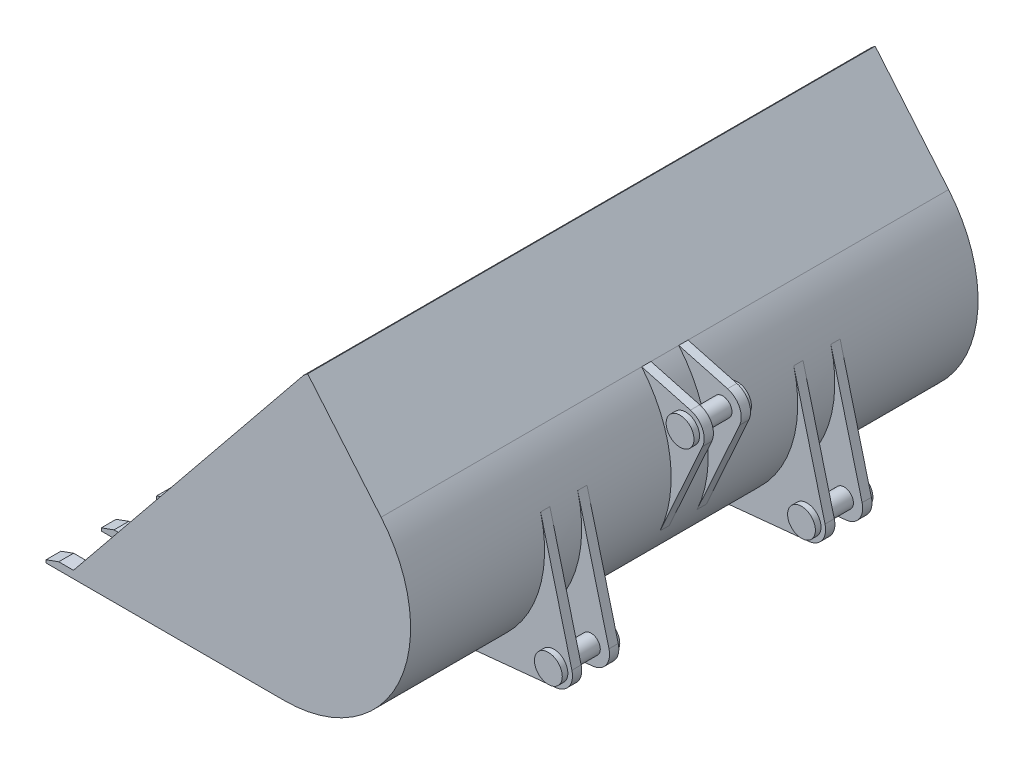
from build123d import *

# Parameters (mm, degrees)
BOSS_EXTRUDE1_DEPTH  = 3000
BOSS_EXTRUDE2_START  = 30
BOSS_EXTRUDE2_DEPTH  = 30
BOSS_EXTRUDE4_START  = -3000
BOSS_EXTRUDE4_DEPTH  = 30
BOSS_EXTRUDE5_START  = -692.5
SKETCH_1_11_R        = 50
BOSS_EXTRUDE5_DEPTH  = 50
BOSS_EXTRUDE6_START  = -892.5
SKETCH_1_12_R        = 50
BOSS_EXTRUDE6_DEPTH  = 50
BOSS_EXTRUDE7_START  = -1375
SKETCH_1_13_2_R      = 50
BOSS_EXTRUDE7_DEPTH  = 50
SKETCH_3_5_R         = 50
BOSS_EXTRUDE8_DEPTH  = 250
BOSS_EXTRUDE9_START  = 30
SKETCH_3_4_R         = 75
SKETCH_3_4_R_2       = 50
BOSS_EXTRUDE9_DEPTH  = 30
BOSS_EXTRUDE10_START = -250
SKETCH_3_5_2_R       = 75
SKETCH_3_5_2_R_2     = 50
BOSS_EXTRUDE10_DEPTH = 30
BOSS_EXTRUDE11_START = 30
SKETCH_4_3_R         = 75
SKETCH_4_3_R_2       = 50
BOSS_EXTRUDE11_DEPTH = 30
SKETCH_4_3_2_R       = 50
BOSS_EXTRUDE12_DEPTH = 125
BOSS_EXTRUDE13_DEPTH = 80
LPATTERN1_COUNT      = 11
LPATTERN1_PITCH      = 298


with BuildPart() as part:
    # Sketch 1_13 → Boss-Extrude1 (new body)
    with BuildSketch(Plane.XY):
        with BuildLine():
            ThreePointArc((1666.98072299, 1087.095574587), (1762.359796854, 362.619582016), (1146.070501669, -30))
            Line((1146.070501669, -30), (0, -30))
            Line((0, -30), (0, 0))
            Line((0, 0), (1146.070501669, 0))
            ThreePointArc((1146.070501669, 0), (1735.170563243, 375.298129869), (1643.999389696, 1067.811946296))
            Line((1643.999389696, 1067.811946296), (1247.99690453, 1539.749330669))
            Line((1247.99690453, 1539.749330669), (1270.978237824, 1559.03295896))
            Line((1270.978237824, 1559.03295896), (1666.98072299, 1087.095574587))
        make_face()
    extrude(amount=-BOSS_EXTRUDE1_DEPTH)

    # 草图1<7> → Boss-Extrude2 (add)
    with BuildSketch(Plane.XY.offset(BOSS_EXTRUDE2_START)):
        with BuildLine():
            Line((1247.99690453, 1539.749330669), (0, 0))
            Line((0, 0), (0, -30))
            Line((0, -30), (1146.070501669, -30))
            ThreePointArc((1146.070501669, -30), (1762.359796854, 362.619582016), (1666.98072299, 1087.095574587))
            Line((1666.98072299, 1087.095574587), (1270.978237824, 1559.03295896))
            Line((1270.978237824, 1559.03295896), (1247.99690453, 1539.749330669))
        make_face()
    extrude(amount=-BOSS_EXTRUDE2_DEPTH)

    # 草图1<9> → Boss-Extrude4 (add)
    with BuildSketch(Plane.XY.offset(BOSS_EXTRUDE4_START)):
        with BuildLine():
            ThreePointArc((1643.999389696, 1067.811946296), (1735.170563243, 375.298129869), (1146.070501669, 0))
            Line((1146.070501669, 0), (0, 0))
            Line((0, 0), (1247.99690453, 1539.749330669))
            Line((1247.99690453, 1539.749330669), (1643.999389696, 1067.811946296))
        make_face()
        with BuildLine():
            ThreePointArc((1666.98072299, 1087.095574587), (1762.359796854, 362.619582016), (1146.070501669, -30))
            Line((1146.070501669, -30), (0, -30))
            Line((0, -30), (0, 0))
            Line((0, 0), (1146.070501669, 0))
            ThreePointArc((1146.070501669, 0), (1735.170563243, 375.298129869), (1643.999389696, 1067.811946296))
            Line((1643.999389696, 1067.811946296), (1247.99690453, 1539.749330669))
            Line((1247.99690453, 1539.749330669), (1270.978237824, 1559.03295896))
            Line((1270.978237824, 1559.03295896), (1666.98072299, 1087.095574587))
        make_face()
    extrude(amount=-BOSS_EXTRUDE4_DEPTH)

    # 草图1<11> → Boss-Extrude5 (add)
    with BuildSketch(Plane.XY.offset(BOSS_EXTRUDE5_START)):
        with BuildLine():
            Line((1213.095596051, -26.688729567), (1886.256631527, 39.986951534))
            ThreePointArc((1886.256631527, 39.986951534), (1958.361695899, 82.208810404), (1973.242532996, 164.430379118))
            Line((1973.242532996, 164.430379118), (1804.599726039, 819.526578004))
            ThreePointArc((1804.599726039, 819.526578004), (1703.410033783, 260.419910747), (1213.095596051, -26.688729567))
        make_face()
        with Locations((1876.4, 139.5)):
            Circle(SKETCH_1_11_R, mode=Mode.SUBTRACT)
    boss_extrude5 = extrude(amount=-BOSS_EXTRUDE5_DEPTH)

    # 草图1<12> → Boss-Extrude6 (add)
    with BuildSketch(Plane.XY.offset(BOSS_EXTRUDE6_START)):
        with BuildLine():
            Line((1213.095596051, -26.688729567), (1886.256631527, 39.986951534))
            ThreePointArc((1886.256631527, 39.986951534), (1958.361695899, 82.208810404), (1973.242532996, 164.430379118))
            Line((1973.242532996, 164.430379118), (1804.599726039, 819.526578004))
            ThreePointArc((1804.599726039, 819.526578004), (1703.410033783, 260.419910747), (1213.095596051, -26.688729567))
        make_face()
        with Locations((1876.4, 139.5)):
            Circle(SKETCH_1_12_R, mode=Mode.SUBTRACT)
    boss_extrude6 = extrude(amount=-BOSS_EXTRUDE6_DEPTH)

    # Sketch 1_13 2 → Boss-Extrude7 (add)
    with BuildSketch(Plane.XY.offset(BOSS_EXTRUDE7_START)):
        with BuildLine():
            Line((1930.061378111, 1016.371252693), (1666.98072299, 1087.095574587))
            ThreePointArc((1666.98072299, 1087.095574587), (1819.685246249, 742.968682279), (1765.902974507, 370.343593645))
            Line((1765.902974507, 370.343593645), (1995.251834241, 878.674057889))
            ThreePointArc((1995.251834241, 878.674057889), (1994.482550811, 962.590121629), (1930.061378111, 1016.371252693))
        make_face()
        with Locations((1904.1, 919.8)):
            Circle(SKETCH_1_13_2_R, mode=Mode.SUBTRACT)
    boss_extrude7 = extrude(amount=-BOSS_EXTRUDE7_DEPTH)

    # Sketch 3_5 → Boss-Extrude8 (add)
    with BuildSketch(Plane.XY.offset(-692.5)):
        with Locations((1876.4, 139.5)):
            Circle(SKETCH_3_5_R)
    boss_extrude8 = extrude(amount=-BOSS_EXTRUDE8_DEPTH)

    # 草图3<4> → Boss-Extrude9 (add)
    # profile 1 of 2: a face of its own
    with BuildSketch(Plane.XY.offset(-692.5).offset(BOSS_EXTRUDE9_START)):
        with Locations((1876.4, 139.5)):
            Circle(SKETCH_3_4_R)
        with Locations((1876.4, 139.5)):
            Circle(SKETCH_3_4_R_2, mode=Mode.SUBTRACT)
    # profile 2 of 2: a face of its own
    with BuildSketch(Plane.XY.offset(-692.5).offset(BOSS_EXTRUDE9_START)):
        with Locations((1876.4, 139.5)):
            Circle(SKETCH_3_4_R_2)
    boss_extrude9 = extrude(amount=-BOSS_EXTRUDE9_DEPTH)

    # Sketch 3_5 2 → Boss-Extrude10 (add)
    # profile 1 of 2: a face of its own
    with BuildSketch(Plane.XY.offset(-692.5).offset(BOSS_EXTRUDE10_START)):
        with Locations((1876.4, 139.5)):
            Circle(SKETCH_3_5_2_R)
        with Locations((1876.4, 139.5)):
            Circle(SKETCH_3_5_2_R_2, mode=Mode.SUBTRACT)
    # profile 2 of 2: a face of its own
    with BuildSketch(Plane.XY.offset(-692.5).offset(BOSS_EXTRUDE10_START)):
        with Locations((1876.4, 139.5)):
            Circle(SKETCH_3_5_2_R_2)
    boss_extrude10 = extrude(amount=-BOSS_EXTRUDE10_DEPTH)

    # Sketch 4_3 → Boss-Extrude11 (add)
    # profile 1 of 2: a face of its own
    with BuildSketch(Plane.XY.offset(-1375).offset(BOSS_EXTRUDE11_START)):
        with Locations((1904.1, 919.8)):
            Circle(SKETCH_4_3_R)
        with Locations((1904.1, 919.8)):
            Circle(SKETCH_4_3_R_2, mode=Mode.SUBTRACT)
    # profile 2 of 2: a face of its own
    with BuildSketch(Plane.XY.offset(-1375).offset(BOSS_EXTRUDE11_START)):
        with Locations((1904.1, 919.8)):
            Circle(SKETCH_4_3_R_2)
    boss_extrude11 = extrude(amount=-BOSS_EXTRUDE11_DEPTH)

    # Sketch 4_3 2 → Boss-Extrude12 (add)
    with BuildSketch(Plane.XY.offset(-1375)):
        with Locations((1904.1, 919.8)):
            Circle(SKETCH_4_3_2_R)
    boss_extrude12 = extrude(amount=-BOSS_EXTRUDE12_DEPTH)

    # Mirror1: Boss-Extrude5, Boss-Extrude6, Boss-Extrude7, Boss-Extrude8, Boss-Extrude9, Boss-Extrude10, Boss-Extrude11, Boss-Extrude12 across plane
    add(boss_extrude5.mirror(Plane.XY.offset(-1500)))
    add(boss_extrude6.mirror(Plane.XY.offset(-1500)))
    add(boss_extrude7.mirror(Plane.XY.offset(-1500)))
    add(boss_extrude8.mirror(Plane.XY.offset(-1500)))
    add(boss_extrude9.mirror(Plane.XY.offset(-1500)))
    add(boss_extrude10.mirror(Plane.XY.offset(-1500)))
    add(boss_extrude11.mirror(Plane.XY.offset(-1500)))
    add(boss_extrude12.mirror(Plane.XY.offset(-1500)))

    # Sketch5 → Boss-Extrude13 (add)
    with BuildSketch(Plane.XY.offset(30)):
        Polygon((0, -30), (-140, -30), (-140, -15), (-71.313064514, 10), (30, 10), (30, -30), align=None)
    boss_extrude13 = extrude(amount=-BOSS_EXTRUDE13_DEPTH)

    # LPattern1: Boss-Extrude13 ×11
    with Locations(*[(0, 0, -i * LPATTERN1_PITCH) for i in range(1, LPATTERN1_COUNT)]):
        add(boss_extrude13)


solid = part.part
